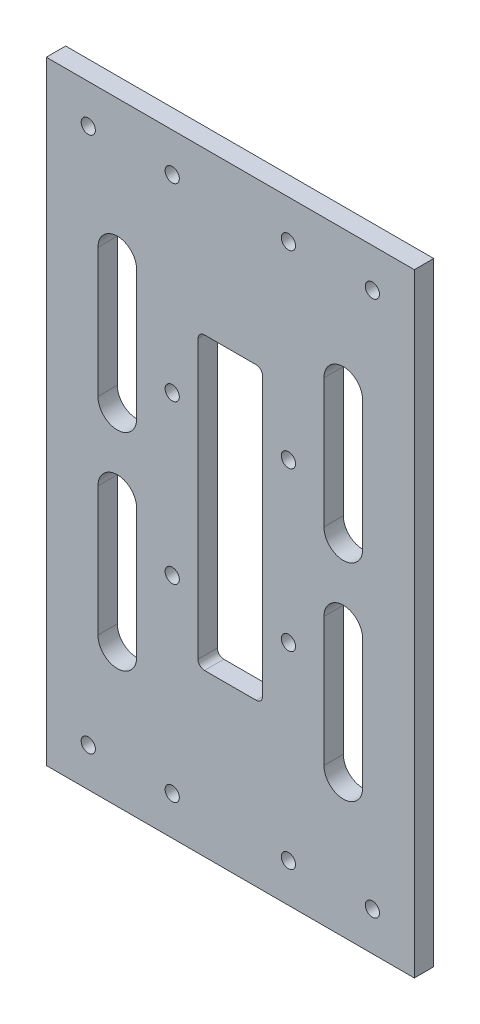
SolidWorks part; units mm, degrees
material "普通碳钢"
ref_plane "前视基准面" through (0, 0, 0) normal (0, 0, 1) x (1, 0, 0)
ref_plane "上视基准面" through (0, 0, 0) normal (0, 1, 0) x (1, 0, 0)
ref_plane "右视基准面" through (0, 0, 0) normal (1, 0, 0) x (0, 0, -1)
sketch "草图1" plane through (0, 0, 0) normal (0, 0, 1) x (1, 0, 0)
  line L1 (1515, 1725) -> (2085, 1725)
  line L2 (1515, 1725) -> (1515, 775)
  line L3 (1515, 775) -> (2085, 775)
  line L4 (2085, 1725) -> (2085, 775)
  line L6 (1515, 1250) -> (2085, 1250) construction
  line L7 (1800, 1725) -> (1800, 775) construction
  line L8 (1625, 1510) -> (1625, 1310) construction
  line L9 (1840, 1025) -> (1760, 1025)
  line L10 (1850, 1035) -> (1850, 1465)
  line L11 (1840, 1475) -> (1760, 1475)
  line L12 (1750, 1035) -> (1750, 1465)
  line L13 (1850, 1025) -> (1750, 1475) construction
  line L14 (1850, 1475) -> (1750, 1025) construction
  line L15 (1655, 1510) -> (1655, 1310)
  line L16 (1595, 1510) -> (1595, 1310)
  line L17 (1975, 1510) -> (1975, 1310) construction
  line L18 (2005, 1510) -> (2005, 1310)
  line L19 (1945, 1510) -> (1945, 1310)
  line L22 (2085, 50) -> (2085, 2450) construction
  line L23 (1515, 50) -> (1515, 2450) construction
  line L24 (1975, 990) -> (1975, 1190) construction
  line L25 (2005, 990) -> (2005, 1190)
  line L26 (1945, 990) -> (1945, 1190)
  line L27 (1625, 990) -> (1625, 1190) construction
  line L28 (1655, 990) -> (1655, 1190)
  line L29 (1595, 990) -> (1595, 1190)
  line L30 (1625, 1310) -> (1625, 1250) construction
  line L31 (1625, 1250) -> (1625, 1190) construction
  circle A0 centre (1580, 1665) radius 11
  circle A1 centre (1710, 1665) radius 11
  circle A2 centre (1890, 1665) radius 11
  circle A3 centre (2020, 1665) radius 11
  arc A4 (1655, 1510) -> (1595, 1510) centre (1625, 1510) ccw
  arc A5 (1595, 1310) -> (1655, 1310) centre (1625, 1310) ccw
  arc A6 (2005, 1510) -> (1945, 1510) centre (1975, 1510) ccw
  arc A7 (1945, 1310) -> (2005, 1310) centre (1975, 1310) ccw
  circle A8 centre (1710, 1372.5) radius 11
  circle A9 centre (1890, 1372.5) radius 11
  circle A10 centre (1710, 1127.5) radius 11
  circle A11 centre (1890, 1127.5) radius 11
  circle A12 centre (2020, 835) radius 11
  circle A13 centre (1890, 835) radius 11
  circle A14 centre (1710, 835) radius 11
  circle A15 centre (1580, 835) radius 11
  arc A16 (1760, 1025) -> (1750, 1035) centre (1760, 1035) cw
  arc A17 (1840, 1025) -> (1850, 1035) centre (1840, 1035) ccw
  arc A18 (1850, 1465) -> (1840, 1475) centre (1840, 1465) ccw
  arc A19 (1760, 1475) -> (1750, 1465) centre (1760, 1465) ccw
  arc A24 (2005, 990) -> (1945, 990) centre (1975, 990) cw
  arc A25 (1945, 1190) -> (2005, 1190) centre (1975, 1190) cw
  arc A26 (1655, 990) -> (1595, 990) centre (1625, 990) cw
  arc A27 (1595, 1190) -> (1655, 1190) centre (1625, 1190) cw
  arc A30 (1655, 1190) -> (1595, 1190) centre (1625, 1190) ccw construction
  point P19 (1800, 1250)
  point P24 (1625, 1410)
  point P33 (1975, 1410)
  point P44 (1975, 1090)
  point P73 (2085, 1250)
  point P81 (1625, 1090)
  dimension "D8" = 22
  dimension "D13" = 10
  dimension "D1" = 950
  dimension "D2" = 60
  dimension "D3" = 130
  dimension "D4" = 60
  dimension "D6" = 100
  dimension "D7" = 450
  dimension "D10" = 440
  dimension "D11" = 122.5
  dimension "D12" = 415
extrude "凸台-拉伸1" add sketch "草图1" along normal blind 30
